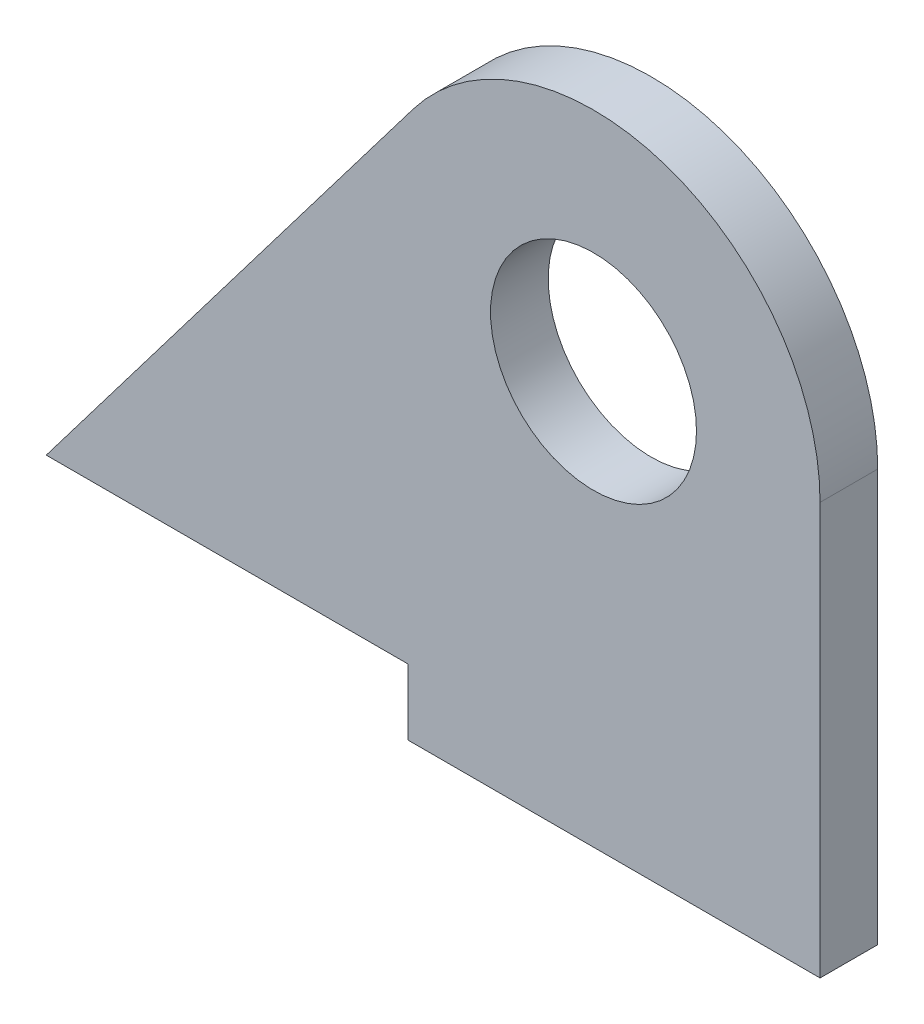
SolidWorks part; units mm, degrees
ref_plane "Front Plane" through (0, 0, 0) normal (0, 0, 1) x (1, 0, 0)
ref_plane "Top Plane" through (0, 0, 0) normal (0, 1, 0) x (1, 0, 0)
ref_plane "Right Plane" through (0, 0, 0) normal (1, 0, 0) x (0, 0, -1)
sketch "Sketch1" plane through (0, 0, 0) normal (0, 0, 1) x (1, 0, 0)
  line L0 (-43.8018, 33.2626) -> (-145, -100)
  line L1 (-145, -100) -> (55, -100)
  line L3 (55, 0) -> (55, -100)
  arc A0 (55, 0) -> (-43.8018, 33.2626) centre (0, 0) ccw
  circle A1 centre (0, 0) radius 25
  dimension "D1" = 50
  dimension "D2" = 110
  dimension "D4" = 145
  dimension "D3" = 100
extrude "Boss-Extrude1" add sketch "Sketch1" along normal blind 14
sketch "Sketch2" plane through (0, 0, 14) normal (0, 0, 1) x (1, 0, 0)
  line L1 (-145, -100) -> (-45, -100)
  line L2 (-145, -100) -> (-145, -84)
  line L3 (-145, -84) -> (-45, -84)
  line L4 (-45, -100) -> (-45, -84)
  dimension "D1" = 16
  dimension "D2" = 100
extrude "Cut-Extrude1" cut sketch "Sketch2" against normal through all
